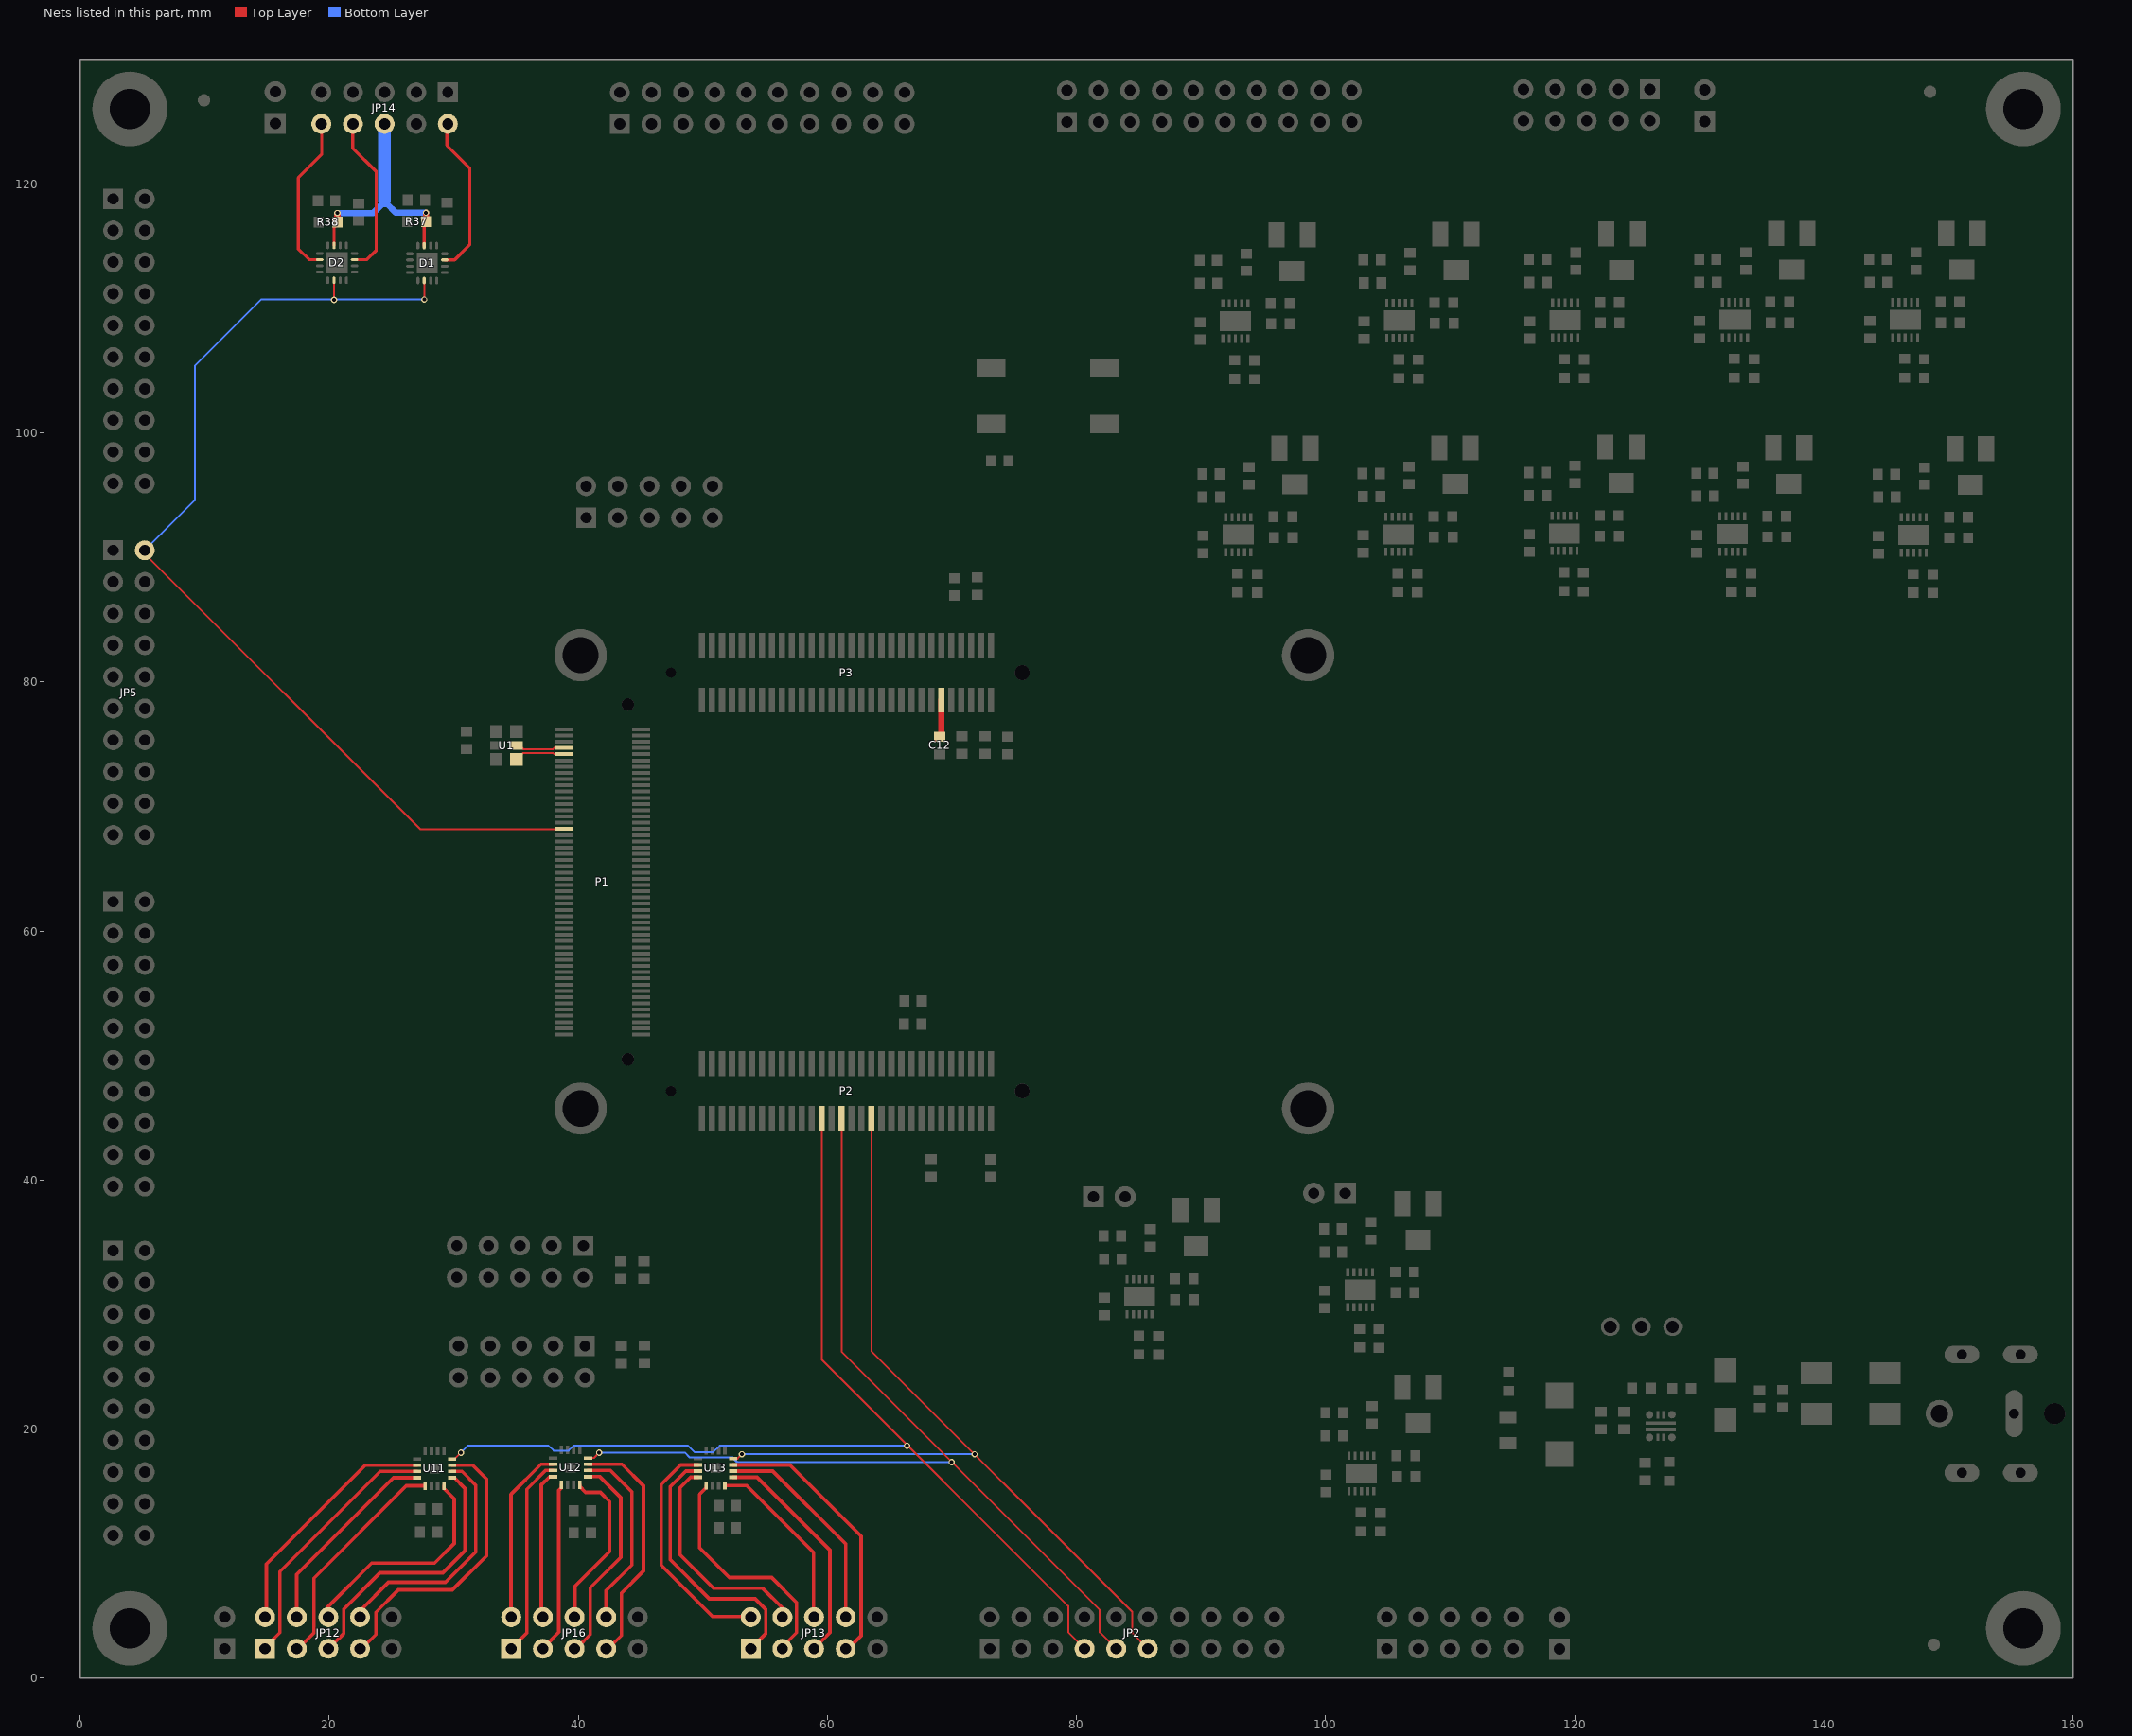
[diagram p0: the nets of this part, all layers, seen from the top]
# Altium PCB MISC82195.PcbDoc (part 3 of 8)
Units mm, origin at the board's own origin, x right, y up, seen from the top; angles counter-clockwise.
Board outline 160 x 130 mm, 4 copper layers (Top Layer, GND, POWER, Bottom Layer); 214 components, 251 nets, 1068 pads, 1218 vias.

## Via types
v1: diameter 0.508, hole 0.305, Top Layer to Bottom Layer, 1218 vias

## Nets (pads, with @x,y where several pads share a name; then routed paths per layer and width w, separated by ;. In a path a pad name is that pad's centre, name@x,y a point inside that pad or via, vN(x,y) a via of type N, cw(c..) or ccw(c..) an arc to the next point about the centre after c; other vN are vias at no path point) (continued)
CDAC1_OUT1: D1.11 JP14.2 | length 12.6
  Top Layer w0.254: D1.11@29.28,113.874 30.08,113.874 31.293,115.087 31.293,121.26 30.188,122.364 29.464,123.088 JP14.2@29.464,124.409
CDAC2_OUT0: D2.2 JP14.10 | length 12.3
  Top Layer w0.254: D2.2@19.241,113.9 18.383,113.9 17.526,114.757 17.526,120.472 19.406,122.352 JP14.10@19.406,124.231
CDAC2_OUT1: D2.11 JP14.8 | length 12.6
  Top Layer w0.254: JP14.8@21.895,124.409 21.895,122.86 23.774,120.98 23.774,114.63 23.044,113.9 D2.11@22.041,113.9
CDAC_VDD: D1.15 D2.15 JP14.6 R37.2 R38.2 | length 18.6
  Top Layer w0.254: D2.15@20.391,115.05 20.391,116.454 R38.2@20.701,116.764 ; D1.15@27.63,115.024 R37.2@27.63,116.591
  Top Layer w0.508: R38.2@20.658,116.926 v1(20.658,117.645) ; R37.2@27.77,116.952 v1(27.77,117.671)
  Bottom Layer w0.508: v1(20.658,117.645) 23.538,117.645 24.384,118.491 ; 24.587,118.44 25.357,117.671 v1(27.77,117.671)
  Bottom Layer w1.016: 24.451,118.609 JP14.6@24.451,124.8
CS_CDAC1: D1.6 D2.6 JP5.2 P1.B34 | length 83.6
  Top Layer w0.152: JP5.2@5.198,90.561 5.198,90.281 27.305,68.174 37.389,68.174 ; v1(20.391,110.663) D2.6@20.391,112.25 ; v1@27.63,110.739 D1.6@27.63,112.224 ; 37.897,68.174 37.389,68.174 ; P1.B34@38.633,68.174 37.389,68.174
  Bottom Layer w0.152: JP5.2@5.198,90.561 6.518,91.882 9.22,94.584 9.22,105.385 14.529,110.693 v1(27.635,110.693)
CS_DAC1: JP2.7 P2.A26 U11.12 | length 90.2
  Top Layer w0.152: U11.12@29.872,17.6 30.072,17.6 v1(30.582,18.11) ; P2.A26@59.537,44.938 59.563,44.913 59.563,43.078 ; 59.563,43.71 59.563,43.078 ; JP2.7@80.645,2.362 79.324,3.683 79.324,5.791 59.563,25.552 59.563,43.078
  Bottom Layer w0.152: v1(30.582,18.11) 31.14,18.669 37.617,18.669 38.024,18.263 39.218,18.263 39.624,18.669 48.819,18.669 49.327,18.161 50.851,18.161 51.359,18.669 58.293,18.669 ; 58.852,18.669 58.293,18.669 ; v1(66.396,18.669) 58.293,18.669
CS_DAC2: JP2.9 P2.A30 U12.12 | length 81.8
  Top Layer w0.152: U12.12@40.794,17.677 41.248,17.677 v1(41.681,18.11) ; 61.138,43.71 61.138,43.256 ; P2.A30@61.138,44.938 61.138,43.256 ; JP2.9@83.185,2.362 81.864,3.683 81.864,5.486 61.138,26.213 61.138,43.256
  Bottom Layer w0.152: v1(41.681,18.11) 48.565,18.11 48.946,17.729 52.375,17.729 52.756,17.348 v1(69.977,17.348)
CS_DAC3: JP2.11 P2.A36 U13.12 | length 71.3
  Top Layer w0.152: U13.12@52.427,17.626 52.779,17.626 v1(53.137,17.983) ; P2.A36@63.537,44.938 63.525,44.926 63.525,26.264 84.48,5.309 84.48,3.607 JP2.11@85.725,2.362
  Bottom Layer w0.152: v1(53.137,17.983) 71.171,17.983 v1(71.806,17.983)
DAC1_OUT0: JP12.2 U11.2 | length 19.1
  Top Layer w0.279: JP12.2@14.961,5.461 14.961,9.169 22.892,17.1 U11.2@27.057,17.1
DAC1_OUT1: JP12.1 U11.3 | length 20.9
  Top Layer w0.279: JP12.1@15.265,2.87 16.053,3.658 16.053,4.445 ; 16.053,3.912 16.053,4.445 ; U11.3@27.057,16.6 24.093,16.6 16.053,8.56 16.053,4.445
DAC1_OUT2: JP12.4 U11.4 | length 16.3
  Top Layer w0.279: JP12.4@17.399,4.902 17.399,8.331 25.168,16.1 U11.4@27.057,16.1
DAC1_OUT3: JP12.3 U11.5 | length 17.8
  Top Layer w0.279: JP12.3@17.755,2.616 18.771,3.632 18.771,8.026 26.187,15.443 U11.5@27.714,15.443
DAC1_OUT4: JP12.6 U11.8 | length 18
  Top Layer w0.279: JP12.6@19.939,4.902 19.939,5.766 23.419,9.246 28.473,9.246 30.048,10.82 30.048,14.402 29.214,15.236 U11.8@29.214,15.443
DAC1_OUT5: JP12.5 U11.9 | length 21.3
  Top Layer w0.279: JP12.5@20.244,2.667 21.184,3.607 21.184,5.563 24.079,8.458 29.134,8.458 30.886,10.211 30.886,15.265 30.051,16.1 U11.9@29.872,16.1
DAC1_OUT6: JP12.8 U11.10 | length 18.9
  Top Layer w0.279: JP12.8@22.555,5.486 24.765,7.696 29.337,7.696 31.775,10.135 31.775,15.494 30.669,16.6 U11.10@29.872,16.6
DAC1_OUT7: JP12.7 U11.11 | length 23
  Top Layer w0.279: JP12.7@22.962,2.718 23.749,3.505 23.749,5.283 25.552,7.087 29.896,7.087 32.639,9.83 32.639,15.977 31.515,17.1 U11.11@29.872,17.1
DAC2_OUT0: JP16.2 U12.2 | length 13.9
  Top Layer w0.279: JP16.2@34.595,5.283 34.595,14.757 37.014,17.177 U12.2@37.979,17.177
DAC2_OUT1: JP16.1 U12.3 | length 15.6
  Top Layer w0.279: JP16.1@34.95,2.718 35.865,3.632 35.865,15.164 37.378,16.677 U12.3@37.979,16.677
DAC2_OUT2: JP16.4 U12.4 | length 11.9
  Top Layer w0.279: JP16.4@37.033,5.309 37.033,6.579 ; 37.033,6.071 37.033,6.579 ; U12.4@37.979,16.177 37.69,16.177 37.033,15.519 37.033,6.579
DAC2_OUT3: JP16.3 U12.5 | length 13.4
  Top Layer w0.279: JP16.3@37.363,2.616 38.43,3.683 38.43,15.062 U12.5@38.633,15.265 ; U12.5@38.636,15.265 U12.5@38.636,15.519
DAC2_OUT4: JP16.6 U12.8 | length 14
  Top Layer w0.279: JP16.6@39.751,5.207 39.751,6.833 ; 39.751,6.02 39.751,6.833 ; U12.8@40.136,15.519 40.136,15.363 40.589,14.91 41.783,14.91 42.52,14.173 42.52,10.16 39.751,7.391 39.751,6.833
DAC2_OUT5: JP16.5 U12.9 | length 16.8
  Top Layer w0.279: JP16.5@39.954,2.489 40.97,3.505 40.97,7.264 43.409,9.703 43.409,14.503 41.735,16.177 U12.9@40.794,16.177
DAC2_OUT6: JP16.8 U12.10 | length 15.4
  Top Layer w0.279: U12.10@40.794,16.677 42.582,16.677 44.298,14.961 44.298,9.093 42.215,7.01 42.215,6.68 ; JP16.8@42.215,5.283 42.215,6.68 ; 42.215,5.994 42.215,6.68
DAC2_OUT7: JP16.7 U12.11 | length 19.1
  Top Layer w0.279: U12.11@40.794,17.177 43.504,17.177 45.237,15.443 45.237,8.611 43.459,6.833 43.459,3.429 JP16.7@42.621,2.591
DAC3_OUT0: JP13.2 U13.2 | length 18.8
  Top Layer w0.279: U13.2@49.612,17.126 48.215,17.126 46.66,15.57 46.66,14.91 46.66,14.757 46.66,9.068 50.775,4.953 JP13.2@53.696,4.953
DAC3_OUT1: JP13.1 U13.3 | length 21
  Top Layer w0.279: U13.3@49.612,16.626 48.63,16.626 47.371,15.367 47.371,9.525 50.521,6.375 54.204,6.375 55.042,5.537 55.042,3.556 JP13.1@54.28,2.794
DAC3_OUT2: JP13.4 U13.4 | length 17.7
  Top Layer w0.279: U13.4@49.612,16.126 49.019,16.126 48.184,15.291 48.184,9.906 50.876,7.214 54.813,7.214 56.413,5.613 JP13.4@56.413,5.105
DAC3_OUT3: JP13.3 U13.5 | length 18.7
  Top Layer w0.279: U13.5@50.267,15.291 49.733,14.757 49.733,10.465 52.121,8.077 55.524,8.077 57.531,6.071 57.531,3.658 JP13.3@56.54,2.667 ; U13.5@50.269,15.291 U13.5@50.269,15.468
DAC3_OUT4: JP13.6 U13.8 | length 14
  Top Layer w0.279: U13.8@51.769,15.468 53.518,15.468 58.877,10.109 JP13.6@58.877,5.486
DAC3_OUT5: JP13.5 U13.9 | length 18.1
  Top Layer w0.279: U13.9@52.427,16.126 54.359,16.126 60.198,10.287 60.198,3.658 JP13.5@59.309,2.769
DAC3_OUT6: JP13.8 U13.10 | length 17.5
  Top Layer w0.279: U13.10@52.427,16.626 55.612,16.626 61.468,10.77 61.468,6.426 ; JP13.8@61.443,5.182 61.468,5.207 61.468,6.426 ; 61.468,6.02 61.468,6.426
DAC3_OUT7: JP13.7 U13.11 | length 21.7
  Top Layer w0.279: U13.11@52.427,17.126 56.991,17.126 62.713,11.405 62.713,3.404 JP13.7@61.951,2.642
FPGA_LVDS_N: P1.B8 U1.5 | length 3.6
  Top Layer w0.152: U1.5@35.408,74.778 35.594,74.591 37.968,74.591 38.065,74.688 P1.B8@38.866,74.688
FPGA_LVDS_P: P1.B10 U1.4 | length 3.5
  Top Layer w0.152: U1.4@35.458,74.168 35.576,74.286 37.968,74.286 38.065,74.188 P1.B10@38.866,74.188
FPGA_VBATT: C12.1 P3.C50 | length 2.7
  Top Layer w0.508: C12.1@69.137,75.82 P3.C50@69.137,78.539